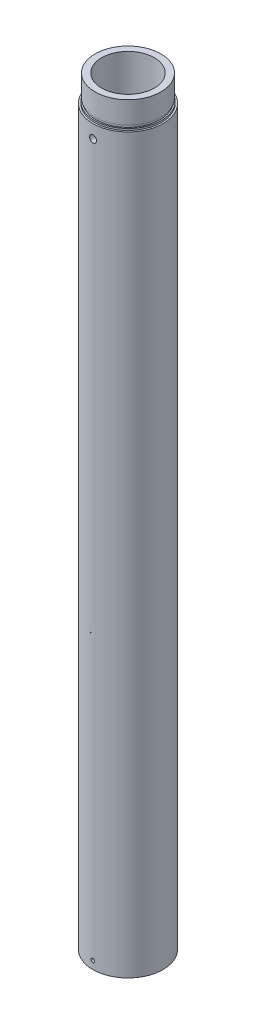
from build123d import *

# Parameters (mm, degrees)
SKETCH1_R             = 40
SKETCH1_R_2           = 30
BOSS_EXTRUDE1_DEPTH   = 864.5
SKETCH2_OUTSIDE_W     = 256.374
SKETCH2_OUTSIDE_H     = 256.374
SKETCH2_OUTSIDE_R     = 37.5
CUT_EXTRUDE1_DEPTH    = 25
SKETCH3_OUTSIDE_W     = 256.374
SKETCH3_OUTSIDE_H     = 256.374
SKETCH3_OUTSIDE_R     = 36.5
CUT_EXTRUDE2_DEPTH    = 3
SKETCH4_OUTSIDE_W     = 256.374
SKETCH4_OUTSIDE_H     = 256.374
SKETCH4_OUTSIDE_R     = 38
CUT_EXTRUDE3_DEPTH    = 2
SKETCH5_R             = 32.5
CUT_EXTRUDE4_DEPTH    = 50
CHAMFER2_SIZE         = 1.5
M5_TAPPED_HOLE1_D     = 4.2
M5_TAPPED_HOLE1_DEPTH = 10
M5_TAPPED_HOLE1_TIP   = 1.2618073
SKETCH8_R             = 4
CUT_EXTRUDE5_DEPTH    = 30


with BuildPart() as part:
    # Sketch1 → Boss-Extrude1 (new body)
    with BuildSketch(Plane(origin=(0, 0, 0), x_dir=(1, 0, 0), z_dir=(0, 1, 0))):
        with Locations(Location((0, 0, 0), (0, 0, 270))):
            Circle(SKETCH1_R)
        with Locations(Location((0, 0, 0), (0, 0, 270))):
            Circle(SKETCH1_R_2, mode=Mode.SUBTRACT)
    extrude(amount=BOSS_EXTRUDE1_DEPTH)

    # Sketch2 outside → Cut-Extrude1 (cut)
    with BuildSketch(Plane(origin=(0, 864.5, 0), x_dir=(1, 0, 0), z_dir=(0, 1, 0))):
        Rectangle(SKETCH2_OUTSIDE_W, SKETCH2_OUTSIDE_H)
        with Locations(Location((0, 0, 0), (0, 0, 270))):
            Circle(SKETCH2_OUTSIDE_R, mode=Mode.SUBTRACT)
    extrude(amount=-CUT_EXTRUDE1_DEPTH, mode=Mode.SUBTRACT)

    # Sketch3 outside → Cut-Extrude2 (cut)
    with BuildSketch(Plane(origin=(0, 839.5, 0), x_dir=(1, 0, 0), z_dir=(0, 1, 0))):
        Rectangle(SKETCH3_OUTSIDE_W, SKETCH3_OUTSIDE_H)
        with Locations(Location((0, 0, 0), (0, 0, 270))):
            Circle(SKETCH3_OUTSIDE_R, mode=Mode.SUBTRACT)
    extrude(amount=-CUT_EXTRUDE2_DEPTH, mode=Mode.SUBTRACT)

    # Sketch4 outside → Cut-Extrude3 (cut)
    with BuildSketch(Plane(origin=(0, 836.5, 0), x_dir=(1, 0, 0), z_dir=(0, 1, 0))):
        Rectangle(SKETCH4_OUTSIDE_W, SKETCH4_OUTSIDE_H)
        with Locations(Location((0, 0, 0), (0, 0, 270))):
            Circle(SKETCH4_OUTSIDE_R, mode=Mode.SUBTRACT)
    extrude(amount=-CUT_EXTRUDE3_DEPTH, mode=Mode.SUBTRACT)

    # Sketch5 → Cut-Extrude4 (cut)
    with BuildSketch(Plane.XZ):
        with Locations(Location((0, 0, 0), (0, 0, 270))):
            Circle(SKETCH5_R)
    extrude(amount=-CUT_EXTRUDE4_DEPTH, mode=Mode.SUBTRACT)

    # Chamfer2
    chamfer2_edges = [part.edges().sort_by_distance(p)[0] for p in [
        (0, 50, -30),
    ]]
    chamfer(chamfer2_edges, length=CHAMFER2_SIZE)

    # M5 Tapped Hole1
    with Locations(Plane.XY.offset(40)):
        with Locations((0, 9)):
            Hole(M5_TAPPED_HOLE1_D / 2, depth=M5_TAPPED_HOLE1_DEPTH)
            with Locations((0, 0, -(M5_TAPPED_HOLE1_DEPTH + M5_TAPPED_HOLE1_TIP / 2))):  # 118° drill point
                Cone(0, M5_TAPPED_HOLE1_D / 2, M5_TAPPED_HOLE1_TIP, mode=Mode.SUBTRACT)

    # Sketch8 → Cut-Extrude5 (cut)
    with BuildSketch(Plane.XY.offset(40)):
        with Locations((0, 819.5)):
            Circle(SKETCH8_R)
    extrude(amount=-CUT_EXTRUDE5_DEPTH, mode=Mode.SUBTRACT)


solid = part.part
